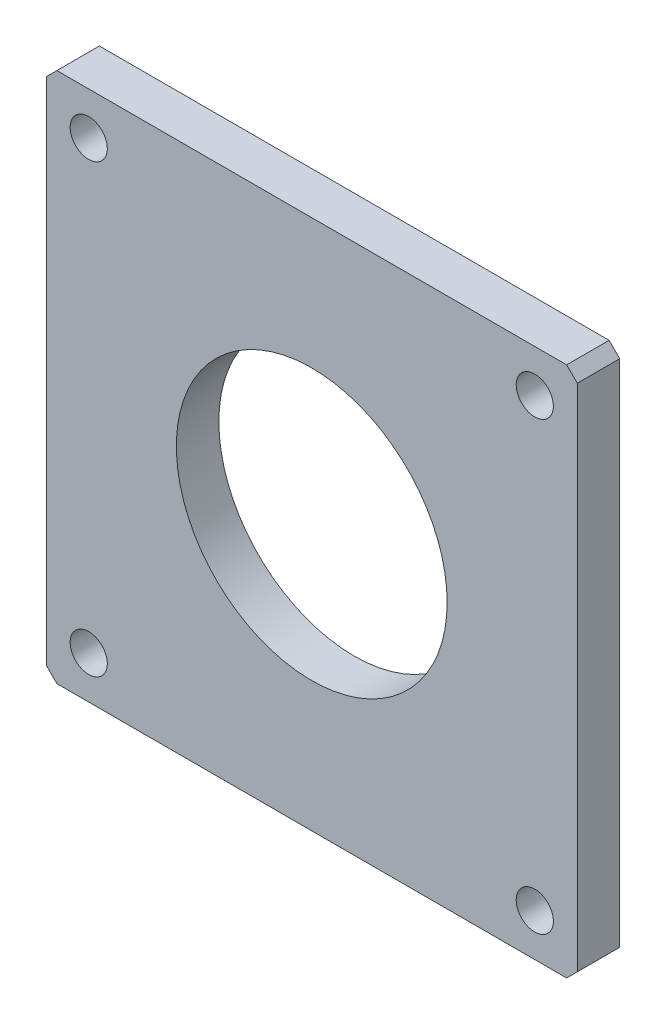
from build123d import *

# Parameters (mm, degrees)
SKETCH_1_W               = 100
SKETCH_1_H               = 100
EXTRUDE_1_DEPTH          = 8
CUT_EXTRUDE_1_REACH      = 73.162
SKETCH_2_R               = 25.5
CUT_EXTRUDE_2_REACH      = 73.162
SKETCH_3_R               = 3.5
PATTERN_CIRCULAR_1_COUNT = 4
CHAMFER_1_SIZE           = 2


with BuildPart() as part:
    # 草图1 → 凸台-拉伸1 (new body)
    with BuildSketch(Plane.XY):
        Rectangle(SKETCH_1_W, SKETCH_1_H)
    extrude(amount=EXTRUDE_1_DEPTH)

    # 草图2 → 切除-拉伸1 (cut, up to next)
    with BuildSketch(Plane.XY.offset(8), mode=Mode.PRIVATE) as cut_extrude_1_sk1:
        Circle(SKETCH_2_R)
    cut_extrude_1_tool1 = extrude(cut_extrude_1_sk1.sketch, amount=-CUT_EXTRUDE_1_REACH, mode=Mode.PRIVATE) & part.part
    add(cut_extrude_1_tool1.solids().sort_by_distance((0, 0, 8))[0], mode=Mode.SUBTRACT)

    # 草图3 → 切除-拉伸2 (cut, up to next)
    with BuildSketch(Plane.XY.offset(8), mode=Mode.PRIVATE) as cut_extrude_2_sk1:
        with Locations((-42, 42)):
            Circle(SKETCH_3_R)
    cut_extrude_2_tool1 = extrude(cut_extrude_2_sk1.sketch, amount=-CUT_EXTRUDE_2_REACH, mode=Mode.PRIVATE) & part.part
    cut_extrude_2 = cut_extrude_2_tool1.solids().sort_by_distance((-42, 42, 8))[0]
    add(cut_extrude_2, mode=Mode.SUBTRACT)

    # 阵列(圆周)1: 切除-拉伸2 ×4 about axis
    pattern_circular_1_axis = Axis((0, 0, 0), (0, 0, 1))
    for i in range(1, PATTERN_CIRCULAR_1_COUNT):
        add(cut_extrude_2.rotate(pattern_circular_1_axis, i * 360 / PATTERN_CIRCULAR_1_COUNT), mode=Mode.SUBTRACT)

    # 倒角1
    chamfer_1_edges = [part.edges().sort_by_distance(p)[0] for p in [
        (50, -50, 4),
        (-50, -50, 4),
        (-50, 50, 4),
        (50, 50, 4),
    ]]
    chamfer(chamfer_1_edges, length=CHAMFER_1_SIZE)


solid = part.part
